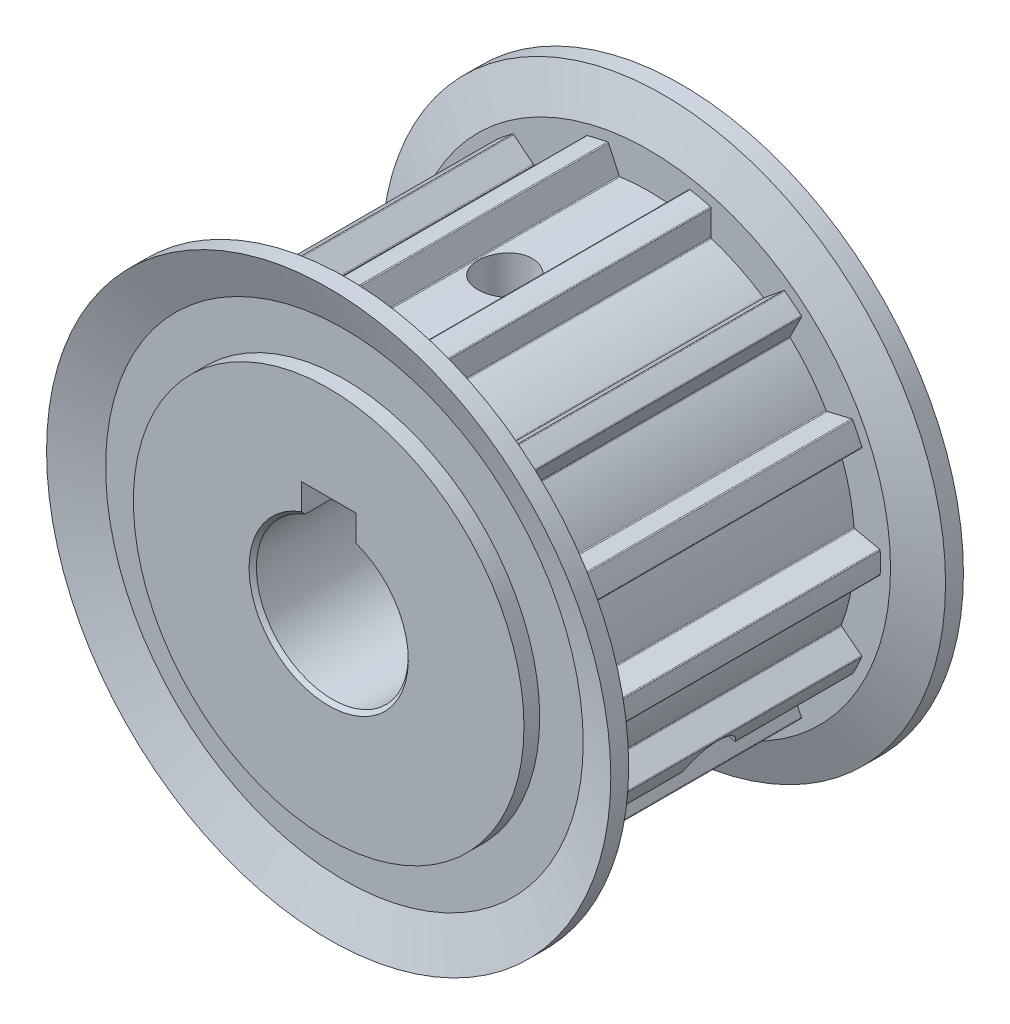
from build123d import *

# Parameters (mm, degrees)
BOSS_EXTRUDE1_DEPTH     = 13.25
CIRPATTERN1_COUNT       = 14
CUT_EXTRUDE2_DEPTH      = 41.20027985
CUT_EXTRUDE2_DEPTH_BACK = 41.20027985
CHAMFER2_SIZE           = 0.34
CUT_EXTRUDE3_START      = 9.3
SKETCH15_R              = 2.5
CUT_EXTRUDE3_DEPTH      = 31.90027985
SKETCH16_R              = 2.5
CUT_EXTRUDE4_DEPTH      = 41.20027985


with BuildPart() as part:
    # Sketch3 → Revolve1 (revolve)
    with BuildSketch(Plane(origin=(0, 0, 0), x_dir=(0, 0, -1), z_dir=(1, 0, 0)), mode=Mode.PRIVATE) as revolve1_sk:
        Polygon((16.25, 0), (16.25, 18), (14.8, 18), (14.8, 22.007265282), (16.25, 26), (14.600953765, 26), (13.25, 22.28), (13.25, 18.99), (-13.25, 18.99), (-13.25, 22.28), (-14.600953765, 26), (-16.25, 26), (-14.8, 22.007265282), (-14.8, 18), (-16.25, 18), (-16.25, 0), align=None)
    revolve(revolve1_sk.sketch.rotate(Axis((0, 0, 16.25), (0, 0, -1)), 90), axis=Axis((0, 0, 16.25), (0, 0, -1)))

    # Sketch4 → Boss-Extrude1 (add, symmetric)
    with BuildSketch(Plane.XY):
        with BuildLine():
            Line((2.736316429, 18.863516323), (3.709155055, 20.94977549))
            ThreePointArc((3.709155055, 20.94977549), (3.753843857, 20.996335591), (3.817667179, 21.005901964))
            ThreePointArc((3.817667179, 21.005901964), (4.75082194, 20.814710925), (5.674520011, 20.582087422))
            ThreePointArc((5.674520011, 20.582087422), (5.727872144, 20.545776516), (5.747933692, 20.484437571))
            Line((5.747933692, 20.484437571), (5.71923708, 18.18268415))
            ThreePointArc((5.71923708, 18.18268415), (5.738091137, 18.122985855), (5.78874618, 18.086196882))
            ThreePointArc((5.78874618, 18.086196882), (4.225672536, 18.513881052), (2.631826637, 18.806743167))
            ThreePointArc((2.631826637, 18.806743167), (2.693427391, 18.817910487), (2.736316429, 18.863516323))
        make_face()
    boss_extrude1 = extrude(amount=BOSS_EXTRUDE1_DEPTH, both=True)

    # CirPattern1: Boss-Extrude1 ×14 about axis
    cirpattern1_axis = Axis((0, 0, 0), (0, 0, 1))
    for i in range(1, CIRPATTERN1_COUNT):
        add(boss_extrude1.rotate(cirpattern1_axis, i * 360 / CIRPATTERN1_COUNT))

    # Sketch9 → Cut-Extrude2 (cut, two sides: drawn at the far end of the back side and taken through both)
    with BuildSketch(Plane.XY.offset(-CUT_EXTRUDE2_DEPTH_BACK)):
        with BuildLine():
            Line((-2.5, 6.538348415), (-2.5, 9.3))
            Line((-2.5, 9.3), (2.5, 9.3))
            Line((2.5, 9.3), (2.5, 6.538348415))
            ThreePointArc((2.5, 6.538348415), (0, -7), (-2.5, 6.538348415))
        make_face()
    extrude(amount=CUT_EXTRUDE2_DEPTH + CUT_EXTRUDE2_DEPTH_BACK, mode=Mode.SUBTRACT)

    # Chamfer2
    chamfer2_edges = [part.edges().sort_by_distance(p)[0] for p in [
        (0, -7, -16.25),
        (0, -7, 16.25),
    ]]
    chamfer(chamfer2_edges, length=CHAMFER2_SIZE)

    # Sketch15 → Cut-Extrude3 (cut, through all)
    with BuildSketch(Plane(origin=(0, 0, 0), x_dir=(1, 0, 0), z_dir=(0, 1, 0)).offset(CUT_EXTRUDE3_START)):
        with Locations(Location((0, 0, 0), (0, 0, 90))):
            Circle(SKETCH15_R)
    extrude(amount=CUT_EXTRUDE3_DEPTH, mode=Mode.SUBTRACT)

    # Sketch16 → Cut-Extrude4 (cut, through all)
    with BuildSketch(Plane(origin=(0, 0, 0), x_dir=(-0.499999999999998, -0.8660254037844398, 0), z_dir=(-0.8660254037844398, 0.499999999999998, 0))):
        Circle(SKETCH16_R)
    extrude(amount=-CUT_EXTRUDE4_DEPTH, mode=Mode.SUBTRACT)


solid = part.part
